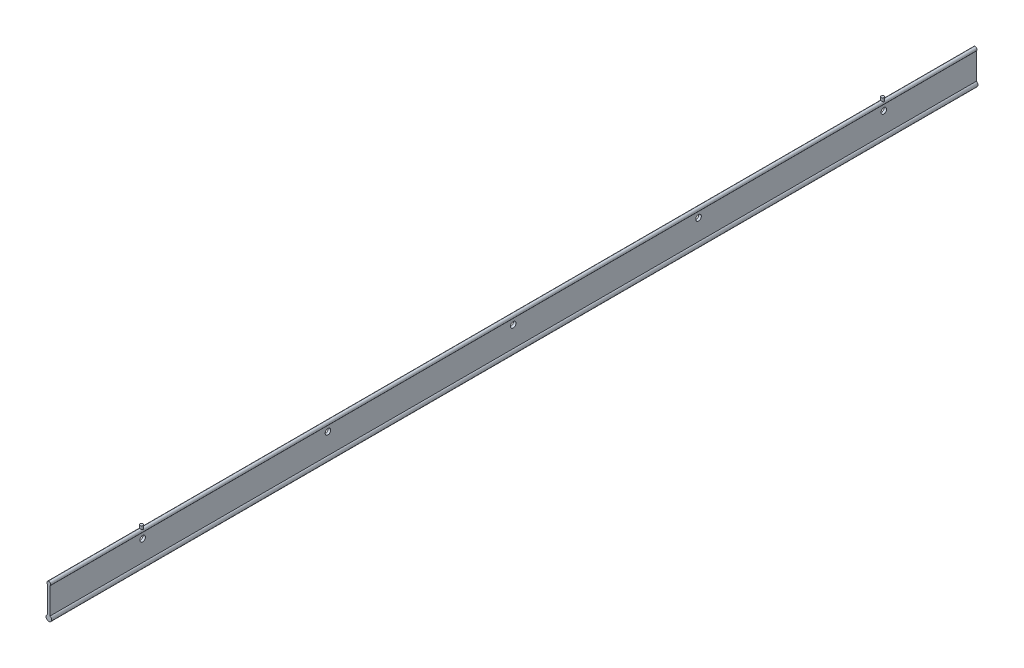
from build123d import *

# Parameters (mm, degrees)
BOSS_EXTRUDE1_DEPTH = 2000
SKETCH2_R           = 6
CUT_EXTRUDE1_DEPTH  = 2002.278667491
SKETCH3_R           = 3.25
BOSS_EXTRUDE2_DEPTH = 10


with BuildPart() as part:
    # Sketch1 → Boss-Extrude1 (new body)
    with BuildSketch(Plane.XY):
        with BuildLine():
            Line((-2.78812886, -2.868159246), (-2.78812886, -59.687153545))
            ThreePointArc((-2.78812886, -59.687153545), (0.061942892, -70.999680248), (2.677842692, -59.630720857))
            Line((2.677842692, -59.630720857), (2.677842692, -2.971389998))
            ThreePointArc((2.677842692, -2.971389998), (0.075530833, 3.999286823), (-2.78812886, -2.868159246))
        make_face()
    extrude(amount=BOSS_EXTRUDE1_DEPTH)

    # Sketch2 → Cut-Extrude1 (cut, through all)
    with BuildSketch(Plane(origin=(2.677842692, 0, 0), x_dir=(0, 0, -1), z_dir=(1, 0, 0))):
        with Locations(Location((-200, -14.971389998, 0), (0, 0, 90))):
            Circle(SKETCH2_R)
        with Locations(Location((-600, -14.971389998, 0), (0, 0, 90))):
            Circle(SKETCH2_R)
        with Locations(Location((-1000, -14.971389998, 0), (0, 0, 90))):
            Circle(SKETCH2_R)
        with Locations(Location((-1400, -14.971389998, 0), (0, 0, 90))):
            Circle(SKETCH2_R)
        with Locations(Location((-1800, -14.971389998, 0), (0, 0, 90))):
            Circle(SKETCH2_R)
    extrude(amount=-CUT_EXTRUDE1_DEPTH, mode=Mode.SUBTRACT)

    # Sketch3 → Boss-Extrude2 (add)
    with BuildSketch(Plane(origin=(0, 0, 0), x_dir=(1, 0, 0), z_dir=(0, 1, 0))):
        with Locations(Location((0, -200, 0), (0, 0, 90))):
            Circle(SKETCH3_R)
        with Locations(Location((0, -1800, 0), (0, 0, 90))):
            Circle(SKETCH3_R)
    extrude(amount=BOSS_EXTRUDE2_DEPTH)


solid = part.part
